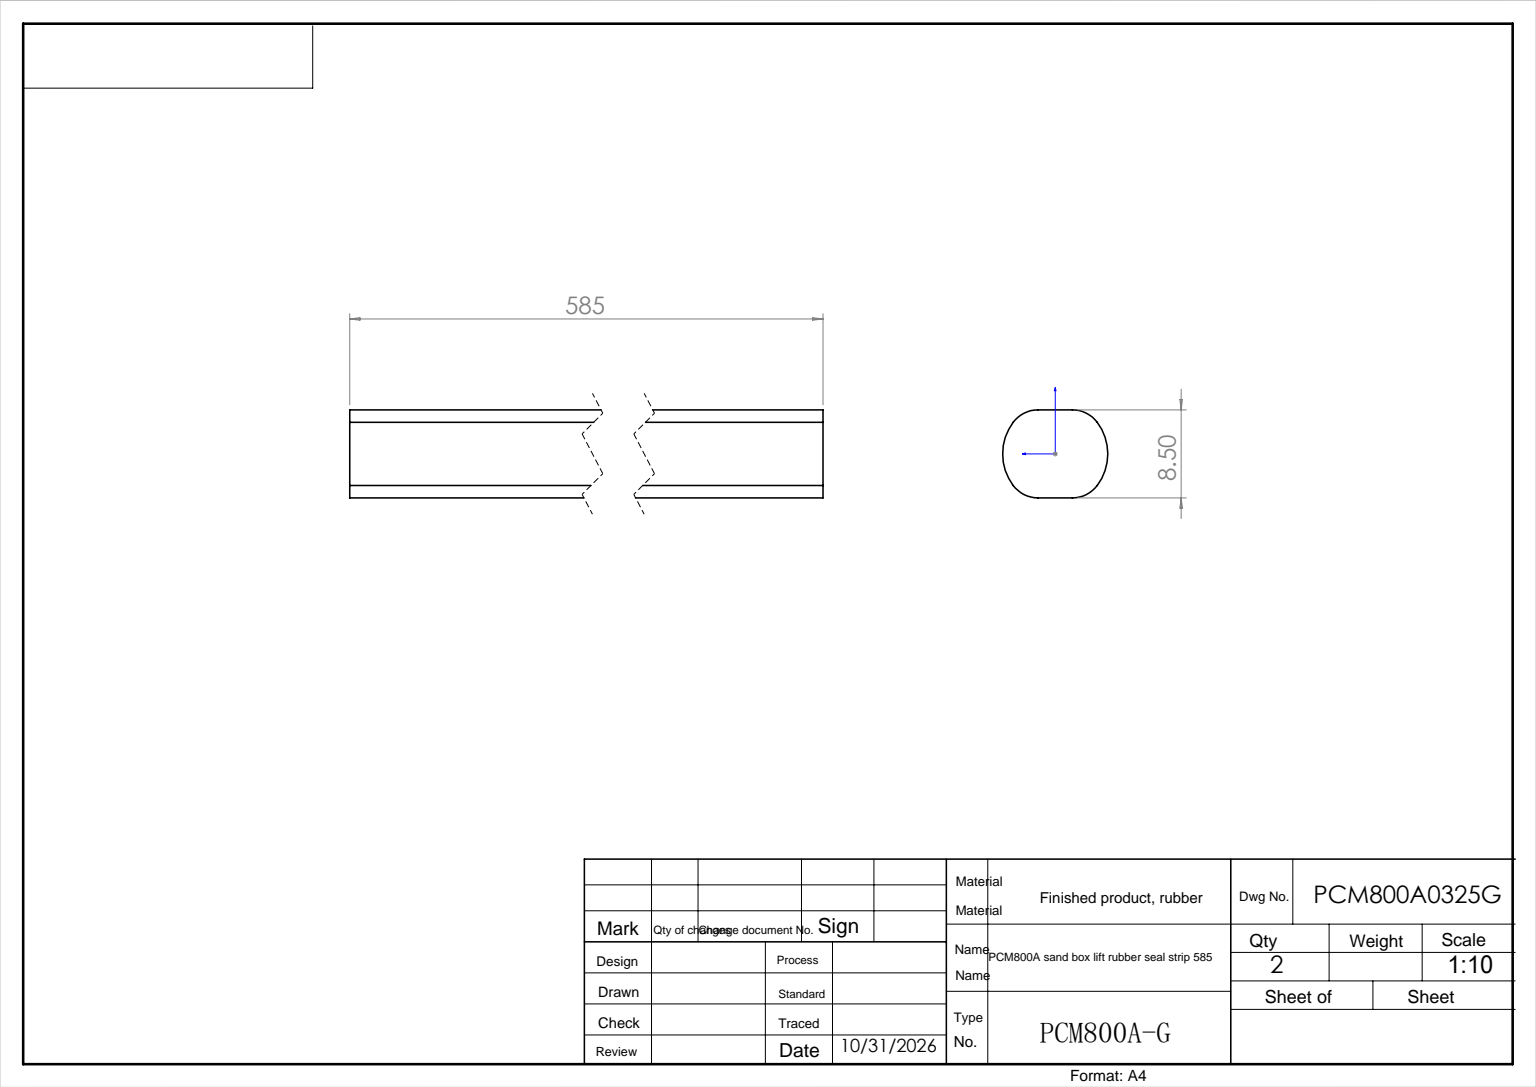
SolidWorks part; units mm, degrees
ref_plane "前视" through (0, 0, 0) normal (0, 0, 1) x (1, 0, 0)
ref_plane "上视" through (0, 0, 0) normal (0, 1, 0) x (1, 0, 0)
ref_plane "右视" through (0, 0, 0) normal (1, 0, 0) x (0, 0, -1)
sketch "草图1" plane through (0, 0, 0) normal (0, 0, 1) x (1, 0, 0)
  line L0 (-1.6615, 4.25) -> (1.6615, 4.25)
  line L1 (-1.6615, -4.25) -> (1.6615, -4.25)
  arc A0 (-4.0588, 3.0536) -> (-4.0588, -3.0536) centre (0, 0) ccw
  arc A1 (4.0588, -3.0536) -> (4.0588, 3.0536) centre (0, 0) ccw
  arc A2 (-4.0588, 3.0536) -> (-1.6615, 4.25) centre (-1.6615, 1.25) cw
  arc A3 (4.0588, 3.0536) -> (1.6615, 4.25) centre (1.6615, 1.25) ccw
  arc A4 (1.6615, -4.25) -> (4.0588, -3.0536) centre (1.6615, -1.25) ccw
  arc A5 (-4.0588, -3.0536) -> (-1.6615, -4.25) centre (-1.6615, -1.25) ccw
  point P10 (2.7813, 4.25)
  point P13 (2.7813, -4.25)
  dimension "D1" = 8.5
  dimension "D3" = 3
  dimension "D2" = 4.25
extrude "拉伸1" add sketch "草图1" along normal blind 585
